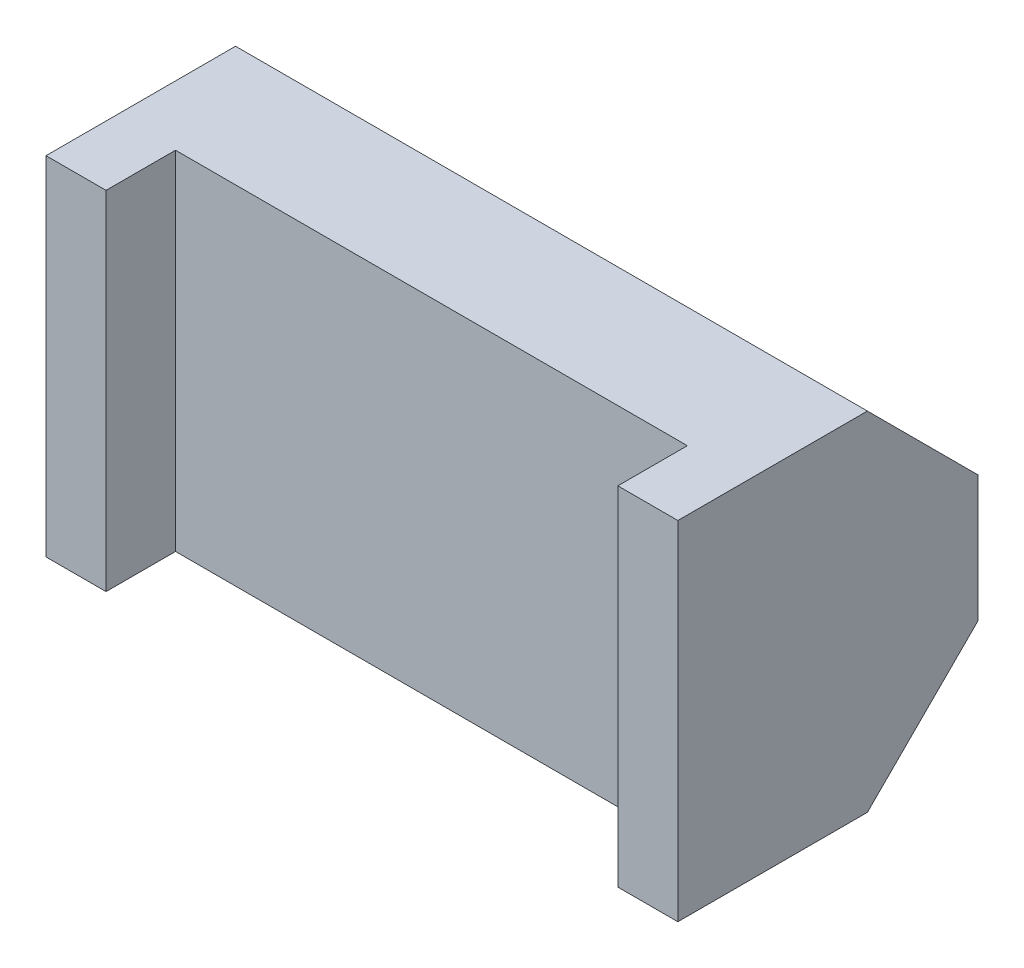
from build123d import *

# Parameters (mm, degrees)
SKETCH_1_W          = 20
SKETCH_1_H          = 11
EXTRUDE_1_DEPTH     = 9.5
SKETCH_2_W          = 16.2
SKETCH_2_H          = 29.89512134
CUT_EXTRUDE_1_DEPTH = 2.2
CUT_EXTRUDE_2_DEPTH = 23.814469093


with BuildPart() as part:
    # 草图1 → 凸台-拉伸1 (new body)
    with BuildSketch(Plane.XY):
        Rectangle(SKETCH_1_W, SKETCH_1_H)
    extrude(amount=EXTRUDE_1_DEPTH)

    # 草图2 → 切除-拉伸1 (cut)
    with BuildSketch(Plane.XY.offset(9.5)):
        Rectangle(SKETCH_2_W, SKETCH_2_H)
    extrude(amount=-CUT_EXTRUDE_1_DEPTH, mode=Mode.SUBTRACT)

    # 草图3 → 切除-拉伸2 (cut, through all)
    with BuildSketch(Plane.ZY.offset(10)):
        Polygon((0, 5.5), (3.5, 5.5), (0, 2), align=None)
    cut_extrude_2 = extrude(amount=-CUT_EXTRUDE_2_DEPTH, mode=Mode.SUBTRACT)

    # 镜向1: 切除-拉伸2 across plane
    add(cut_extrude_2.mirror(Plane.ZX), mode=Mode.SUBTRACT)


solid = part.part
